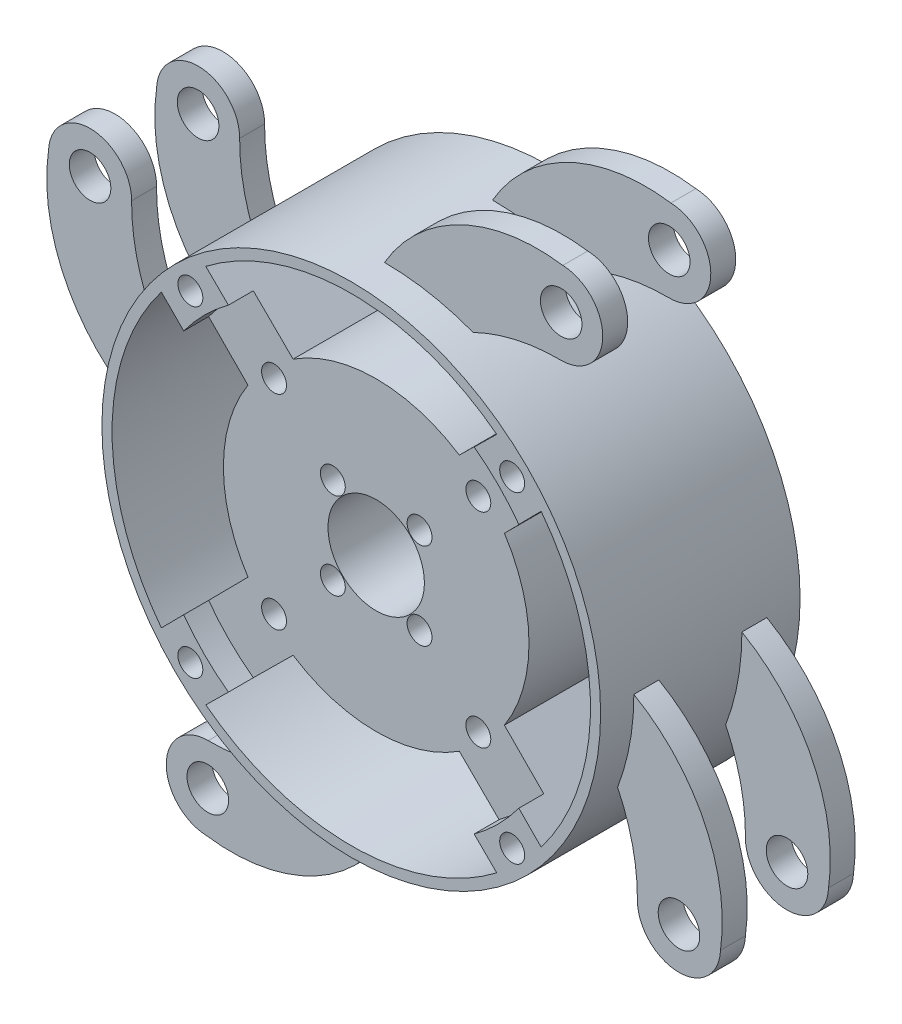
from build123d import *
from build123d.topology import SkipClean

# Parameters (mm, degrees)
SKETCH1_R           = 30
SKETCH1_R_2         = 5.8
BOSS_EXTRUDE1_DEPTH = 12
CUT_EXTRUDE1_DEPTH  = 49.744230428
SKETCH3_R           = 1.5
CUT_EXTRUDE2_DEPTH  = 49.744230428
SKETCH4_R           = 25
CUT_EXTRUDE3_DEPTH  = 3
SKETCH5_R           = 2.5
BOSS_EXTRUDE2_DEPTH = 8
CIRPATTERN1_COUNT   = 4
CUT_EXTRUDE11_DEPTH = 2.5
SCALE_1_SCALE       = 0.5
CUT_EXTRUDE12_DEPTH = 2.5


with BuildPart() as part:
    # Sketch1 → Boss-Extrude1 (new, symmetric)
    with BuildSketch(Plane.XY):
        Circle(SKETCH1_R)
        Circle(SKETCH1_R_2, mode=Mode.SUBTRACT)
    extrude(amount=BOSS_EXTRUDE1_DEPTH, both=True)

    # Sketch2 → Cut-Extrude1 (cut, through all)
    with BuildSketch(Plane.XY.offset(12)):
        with BuildLine():
            Line((-17.5, 22.846247275), (-10, 15.426831039))
            ThreePointArc((-10, 15.426831039), (0, 18.384425906), (10, 15.426831039))
            Line((10, 15.426831039), (17.5, 22.846247275))
            ThreePointArc((17.5, 22.846247275), (0, 28.778481797), (-17.5, 22.846247275))
        make_face()
        with BuildLine():
            Line((15.426831039, -10), (22.846247275, -17.5))
            ThreePointArc((22.846247275, -17.5), (28.778481797, 0), (22.846247275, 17.5))
            Line((22.846247275, 17.5), (15.426831039, 10))
            ThreePointArc((15.426831039, 10), (18.384425906, 0), (15.426831039, -10))
        make_face()
        with BuildLine():
            Line((-10, -15.426831039), (-17.5, -22.846247275))
            ThreePointArc((-17.5, -22.846247275), (0, -28.778481797), (17.5, -22.846247275))
            Line((17.5, -22.846247275), (10, -15.426831039))
            ThreePointArc((10, -15.426831039), (0, -18.384425906), (-10, -15.426831039))
        make_face()
        with BuildLine():
            Line((-15.426831039, 10), (-22.846247275, 17.5))
            ThreePointArc((-22.846247275, 17.5), (-28.778481797, 0), (-22.846247275, -17.5))
            Line((-22.846247275, -17.5), (-15.426831039, -10))
            ThreePointArc((-15.426831039, -10), (-18.384425906, 0), (-15.426831039, 10))
        make_face()
    extrude(amount=-CUT_EXTRUDE1_DEPTH, mode=Mode.SUBTRACT)

    # Sketch3 → Cut-Extrude2 (cut, through all)
    with BuildSketch(Plane.XY.offset(12)):
        with Locations((-19.358791633, 19.358791633)):
            Circle(SKETCH3_R)
        with Locations((-12.287723821, 12.287723821)):
            Circle(SKETCH3_R)
        with Locations((-5.216656009, 5.216656009)):
            Circle(SKETCH3_R)
        with Locations((19.358791633, 19.358791633)):
            Circle(SKETCH3_R)
        with Locations((12.287723821, 12.287723821)):
            Circle(SKETCH3_R)
        with Locations((5.216656009, 5.216656009)):
            Circle(SKETCH3_R)
        with Locations((19.358791633, -19.358791633)):
            Circle(SKETCH3_R)
        with Locations((12.287723821, -12.287723821)):
            Circle(SKETCH3_R)
        with Locations((5.216656009, -5.216656009)):
            Circle(SKETCH3_R)
        with Locations((-19.358791633, -19.358791633)):
            Circle(SKETCH3_R)
        with Locations((-12.287723821, -12.287723821)):
            Circle(SKETCH3_R)
        with Locations((-5.216656009, -5.216656009)):
            Circle(SKETCH3_R)
    extrude(amount=-CUT_EXTRUDE2_DEPTH, mode=Mode.SUBTRACT)

    # Sketch4 → Cut-Extrude3 (cut)
    with BuildSketch(Plane.XY.offset(12)):
        Circle(SKETCH4_R)
    cut_extrude3 = extrude(amount=-CUT_EXTRUDE3_DEPTH, mode=Mode.SUBTRACT)

    # Mirror1: Cut-Extrude3 across plane
    add(cut_extrude3.mirror(Plane.XY), mode=Mode.SUBTRACT)

    # Sketch5 → Boss-Extrude2 (add, symmetric)
    with BuildSketch(Plane.XY):
        with BuildLine():
            ThreePointArc((0, 30), (9.130183529, 38.500591706), (21.455952915, 40.423017172))
            ThreePointArc((21.455952915, 40.423017172), (26.256509779, 35.30886651), (21.219834085, 30.427085978))
            ThreePointArc((21.219834085, 30.427085978), (15.801391202, 29.844023046), (10.657871278, 28.042998767))
            ThreePointArc((10.657871278, 28.042998767), (5.418027178, 29.506693842), (0, 30))
        make_face()
        with Locations((21.257904133, 35.426941044)):
            Circle(SKETCH5_R, mode=Mode.SUBTRACT)
    boss_extrude2 = extrude(amount=BOSS_EXTRUDE2_DEPTH, both=True)

    # CirPattern1: Boss-Extrude2 ×4 about axis
    cirpattern1_axis = Axis((0, 0, 0), (0, 0, 1))
    for i in range(1, CIRPATTERN1_COUNT):
        add(boss_extrude2.rotate(cirpattern1_axis, i * 360 / CIRPATTERN1_COUNT))

    # Sketch16 → Cut-Extrude11 (cut, symmetric)
    with SkipClean():  # the faces are left unmerged after this step: merging them gives an invalid solid
        with BuildSketch(Plane.XY):
            with BuildLine():
                ThreePointArc((-10.657871278, -28.042998767), (-5.418027178, -29.506693842), (0, -30))
                ThreePointArc((0, -30), (-9.130183529, -38.500591706), (-21.455952915, -40.423017172))
                ThreePointArc((-21.455952915, -40.423017172), (-26.256509779, -35.30886651), (-21.219834085, -30.427085978))
                ThreePointArc((-21.219834085, -30.427085978), (-15.801391202, -29.844023046), (-10.657871278, -28.042998767))
            make_face()
            with BuildLine():
                ThreePointArc((28.042998767, -10.657871278), (29.506693842, -5.418027178), (30, 0))
                ThreePointArc((30, 0), (38.500591706, -9.130183529), (40.423017172, -21.455952915))
                ThreePointArc((40.423017172, -21.455952915), (35.30886651, -26.256509779), (30.427085978, -21.219834085))
                ThreePointArc((30.427085978, -21.219834085), (29.844023046, -15.801391202), (28.042998767, -10.657871278))
            make_face()
            with BuildLine():
                ThreePointArc((10.657871278, 28.042998767), (5.418027178, 29.506693842), (0, 30))
                ThreePointArc((0, 30), (9.130183529, 38.500591706), (21.455952915, 40.423017172))
                ThreePointArc((21.455952915, 40.423017172), (26.256509779, 35.30886651), (21.219834085, 30.427085978))
                ThreePointArc((21.219834085, 30.427085978), (15.801391202, 29.844023046), (10.657871278, 28.042998767))
            make_face()
            with BuildLine():
                ThreePointArc((-28.042998767, 10.657871278), (-29.506693842, 5.418027178), (-30, 0))
                ThreePointArc((-30, 0), (-38.500591706, 9.130183529), (-40.423017172, 21.455952915))
                ThreePointArc((-40.423017172, 21.455952915), (-35.30886651, 26.256509779), (-30.427085978, 21.219834085))
                ThreePointArc((-30.427085978, 21.219834085), (-29.844023046, 15.801391202), (-28.042998767, 10.657871278))
            make_face()
        extrude(amount=CUT_EXTRUDE11_DEPTH, both=True, mode=Mode.SUBTRACT)


with BuildPart() as part_1:
    # Scale 1: scaled about (0, 0, 0)
    add(part.part.scale(SCALE_1_SCALE))

    # Sketch17 → Cut-Extrude12 (cut, symmetric)
    with SkipClean():  # the faces are left unmerged after this step: merging them gives an invalid solid
        with BuildSketch(Plane.XY):
            with BuildLine():
                ThreePointArc((-5.328935639, -14.021499383), (-2.709013589, -14.753346921), (0, -15))
                ThreePointArc((0, -15), (-4.565091764, -19.250295853), (-10.727976457, -20.211508586))
                ThreePointArc((-10.727976457, -20.211508586), (-13.128254889, -17.654433255), (-10.609917043, -15.213542989))
                ThreePointArc((-10.609917043, -15.213542989), (-7.900695601, -14.922011523), (-5.328935639, -14.021499383))
            make_face()
            with BuildLine():
                ThreePointArc((14.021499383, -5.328935639), (14.753346921, -2.709013589), (15, 0))
                ThreePointArc((15, 0), (19.250295853, -4.565091764), (20.211508586, -10.727976457))
                ThreePointArc((20.211508586, -10.727976457), (17.654433255, -13.128254889), (15.213542989, -10.609917043))
                ThreePointArc((15.213542989, -10.609917043), (14.922011523, -7.900695601), (14.021499383, -5.328935639))
            make_face()
            with BuildLine():
                ThreePointArc((5.328935639, 14.021499383), (2.709013589, 14.753346921), (0, 15))
                ThreePointArc((0, 15), (4.565091764, 19.250295853), (10.727976457, 20.211508586))
                ThreePointArc((10.727976457, 20.211508586), (13.128254889, 17.654433255), (10.609917043, 15.213542989))
                ThreePointArc((10.609917043, 15.213542989), (7.900695601, 14.922011523), (5.328935639, 14.021499383))
            make_face()
            with BuildLine():
                ThreePointArc((-14.021499383, 5.328935639), (-14.753346921, 2.709013589), (-15, 0))
                ThreePointArc((-15, 0), (-19.250295853, 4.565091764), (-20.211508586, 10.727976457))
                ThreePointArc((-20.211508586, 10.727976457), (-17.654433255, 13.128254889), (-15.213542989, 10.609917043))
                ThreePointArc((-15.213542989, 10.609917043), (-14.922011523, 7.900695601), (-14.021499383, 5.328935639))
            make_face()
        extrude(amount=CUT_EXTRUDE12_DEPTH, both=True, mode=Mode.SUBTRACT)


solid = part_1.part
